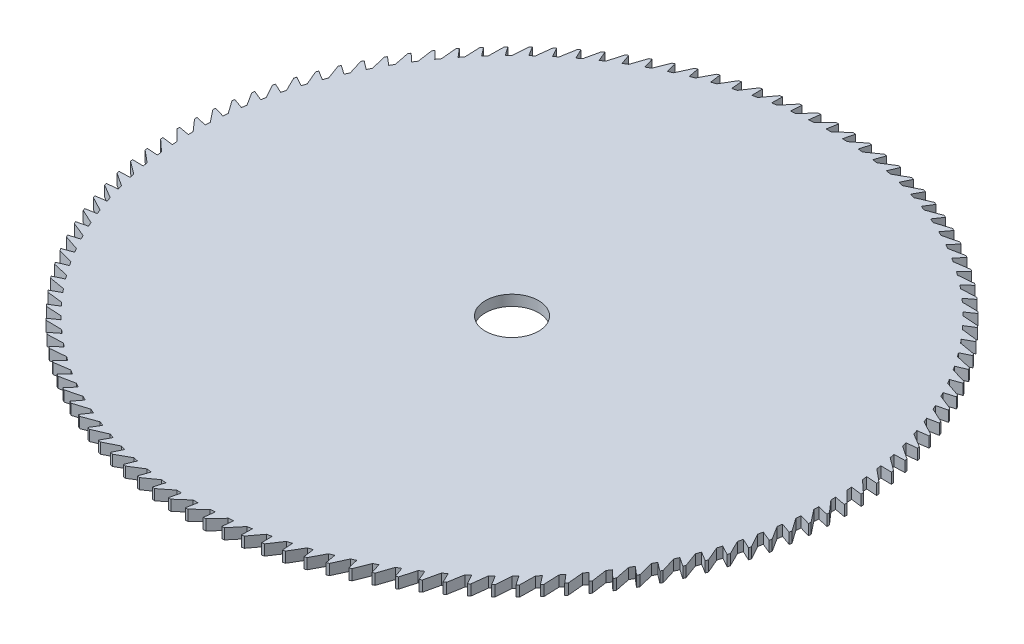
SolidWorks part; units mm, degrees
ref_plane "Front Plane" through (0, 0, 0) normal (0, 0, 1) x (1, 0, 0)
ref_plane "Top Plane" through (0, 0, 0) normal (0, 1, 0) x (1, 0, 0)
ref_plane "Right Plane" through (0, 0, 0) normal (1, 0, 0) x (0, 0, -1)
sketch "Sketch2" plane through (0, 0, 0) normal (0, 1, 0) x (1, 0, 0)
  circle A0 centre (0, 0) radius 150
  circle A1 centre (0, 0) radius 12.5
  dimension "D1" = 25
  dimension "D2" = 300
extrude "Boss-Extrude1" add sketch "Sketch2" along normal blind 5
sketch "Sketch3" plane through (0, 5, 0) normal (0, 1, 0) x (1, 0, 0)
  line L0 (0, 150) -> (0, -150) construction
  line L1 (0, 150) -> (5.59, 154.8992)
  line L2 (6.7665, 154.8522) -> (5.59, 149.8958)
  line L3 (7.8504, 149.7944) -> (13.6891, 154.3943)
  line L4 (14.8616, 154.2859) -> (13.4273, 149.3978)
  line L5 (15.6793, 149.1783) -> (21.7508, 153.4663)
  line L6 (22.9159, 153.2966) -> (21.2278, 148.4903)
  line L7 (23.4652, 148.1533) -> (29.7528, 152.1176)
  line L8 (30.9074, 151.8872) -> (28.9701, 147.1759)
  line L9 (31.1868, 146.7221) -> (37.6732, 150.352)
  line L10 (38.8142, 150.0615) -> (36.6329, 145.458)
  line L11 (38.8229, 144.8889) -> (45.4904, 148.1743)
  line L12 (46.6147, 147.8245) -> (44.1954, 143.3414)
  line L13 (46.3525, 142.6585) -> (53.1829, 145.5905)
  line L14 (54.2873, 145.1823) -> (51.6368, 140.832)
  line L15 (53.7552, 140.0371) -> (60.7296, 142.6076)
  line L16 (61.8112, 142.1421) -> (58.9366, 137.9365)
  line L17 (61.0105, 137.0318) -> (68.1099, 139.2338)
  line L18 (69.1656, 138.7124) -> (66.0748, 134.663)
  line L19 (68.0986, 133.651) -> (75.3035, 135.4784)
  line L20 (76.3304, 134.9024) -> (73.032, 131.0203)
  line L21 (75, 129.9038) -> (82.2907, 131.3516)
  line L22 (83.2861, 130.7227) -> (79.789, 127.0186)
  line L23 (81.6959, 125.8006) -> (89.0523, 126.8648)
  line L24 (90.0134, 126.1847) -> (86.3273, 122.6687)
  line L25 (88.1678, 121.3525) -> (95.5699, 122.0303)
  line L26 (96.4941, 121.3008) -> (92.629, 117.9825)
  line L27 (94.3981, 116.5719) -> (101.8255, 116.8614)
  line L28 (102.7102, 116.0845) -> (98.6767, 112.973)
  line L29 (100.3696, 111.4717) -> (107.802, 111.3721)
  line L30 (108.6449, 110.55) -> (104.4541, 107.6538)
  line L31 (106.066, 106.066) -> (113.483, 105.5775)
  line L32 (114.2817, 104.7124) -> (109.9451, 102.0396)
  line L33 (111.4717, 100.3696) -> (118.853, 99.4936)
  line L34 (119.6053, 98.5879) -> (115.1347, 96.1457)
  line L35 (116.5719, 94.3981) -> (123.8972, 93.137)
  line L36 (124.6011, 92.1931) -> (120.0088, 89.9882)
  line L37 (121.3525, 88.1678) -> (128.6018, 86.525)
  line L38 (129.2553, 85.5456) -> (124.554, 83.5841)
  line L39 (125.8006, 81.6959) -> (132.9539, 79.676)
  line L40 (133.5553, 78.6637) -> (128.7577, 76.9509)
  line L41 (129.9038, 75) -> (136.9416, 72.6085)
  line L42 (137.4892, 71.5662) -> (132.6086, 70.1068)
  line L43 (133.651, 68.0986) -> (140.554, 65.342)
  line L44 (141.0463, 64.2724) -> (136.0959, 63.0705)
  line L45 (137.0318, 61.0105) -> (143.7811, 57.8964)
  line L46 (144.2167, 56.8026) -> (139.2103, 55.8614)
  line L47 (140.0371, 53.7552) -> (146.6141, 50.2922)
  line L48 (146.9919, 49.177) -> (141.9431, 48.4991)
  line L49 (142.6585, 46.3525) -> (149.0453, 42.5501)
  line L50 (149.3642, 41.4166) -> (144.2868, 41.0039)
  line L51 (144.8889, 38.8229) -> (151.0679, 34.6913)
  line L52 (151.3271, 33.5428) -> (146.235, 33.3964)
  line L53 (146.7221, 31.1868) -> (152.6765, 26.7375)
  line L54 (152.8752, 25.5769) -> (147.7824, 25.6972)
  line L55 (148.1533, 23.4652) -> (153.8666, 18.7104)
  line L56 (154.0043, 17.541) -> (148.9248, 17.9277)
  line L57 (149.1783, 15.6793) -> (154.6349, 10.632)
  line L58 (154.7112, 9.457) -> (149.659, 10.109)
  line L59 (149.7944, 7.8504) -> (154.9794, 2.5244)
  line L60 (154.9941, 1.3471) -> (149.9829, 2.2626)
  line L61 (150, 0) -> (154.8992, -5.59)
  line L62 (154.8522, -6.7665) -> (149.8958, -5.59)
  line L63 (149.7944, -7.8504) -> (154.3943, -13.6891)
  line L64 (154.2859, -14.8616) -> (149.3978, -13.4273)
  line L65 (149.1783, -15.6793) -> (153.4663, -21.7508)
  line L66 (153.2966, -22.9159) -> (148.4903, -21.2278)
  line L67 (148.1533, -23.4652) -> (152.1176, -29.7528)
  line L68 (151.8872, -30.9074) -> (147.1759, -28.9701)
  line L69 (146.7221, -31.1868) -> (150.352, -37.6732)
  line L70 (150.0615, -38.8142) -> (145.458, -36.6329)
  line L71 (144.8889, -38.8229) -> (148.1743, -45.4904)
  line L72 (147.8245, -46.6147) -> (143.3414, -44.1954)
  line L73 (142.6585, -46.3525) -> (145.5905, -53.1829)
  line L74 (145.1823, -54.2873) -> (140.832, -51.6368)
  line L75 (140.0371, -53.7552) -> (142.6076, -60.7296)
  line L76 (142.1421, -61.8112) -> (137.9365, -58.9366)
  line L77 (137.0318, -61.0105) -> (139.2338, -68.1099)
  line L78 (138.7124, -69.1656) -> (134.663, -66.0748)
  line L79 (133.651, -68.0986) -> (135.4784, -75.3035)
  line L80 (134.9024, -76.3304) -> (131.0203, -73.032)
  line L81 (129.9038, -75) -> (131.3516, -82.2907)
  line L82 (130.7227, -83.2861) -> (127.0186, -79.789)
  line L83 (125.8006, -81.6959) -> (126.8648, -89.0523)
  line L84 (126.1847, -90.0134) -> (122.6687, -86.3273)
  line L85 (121.3525, -88.1678) -> (122.0303, -95.5699)
  line L86 (121.3008, -96.4941) -> (117.9825, -92.629)
  line L87 (116.5719, -94.3981) -> (116.8614, -101.8255)
  line L88 (116.0845, -102.7102) -> (112.973, -98.6767)
  line L89 (111.4717, -100.3696) -> (111.3721, -107.802)
  line L90 (110.55, -108.6449) -> (107.6538, -104.4541)
  line L91 (106.066, -106.066) -> (105.5775, -113.483)
  line L92 (104.7124, -114.2817) -> (102.0396, -109.9451)
  line L93 (100.3696, -111.4717) -> (99.4936, -118.853)
  line L94 (98.5879, -119.6053) -> (96.1457, -115.1347)
  line L95 (94.3981, -116.5719) -> (93.137, -123.8972)
  line L96 (92.1931, -124.6011) -> (89.9882, -120.0088)
  line L97 (88.1678, -121.3525) -> (86.525, -128.6018)
  line L98 (85.5456, -129.2553) -> (83.5841, -124.554)
  line L99 (81.6959, -125.8006) -> (79.676, -132.9539)
  line L100 (78.6637, -133.5553) -> (76.9509, -128.7577)
  line L101 (75, -129.9038) -> (72.6085, -136.9416)
  line L102 (71.5662, -137.4892) -> (70.1068, -132.6086)
  line L103 (68.0986, -133.651) -> (65.342, -140.554)
  line L104 (64.2724, -141.0463) -> (63.0705, -136.0959)
  line L105 (61.0105, -137.0318) -> (57.8964, -143.7811)
  line L106 (56.8026, -144.2167) -> (55.8614, -139.2103)
  line L107 (53.7552, -140.0371) -> (50.2922, -146.6141)
  line L108 (49.177, -146.9919) -> (48.4991, -141.9431)
  line L109 (46.3525, -142.6585) -> (42.5501, -149.0453)
  line L110 (41.4166, -149.3642) -> (41.0039, -144.2868)
  line L111 (38.8229, -144.8889) -> (34.6913, -151.0679)
  line L112 (33.5428, -151.3271) -> (33.3964, -146.235)
  line L113 (31.1868, -146.7221) -> (26.7375, -152.6765)
  line L114 (25.5769, -152.8752) -> (25.6972, -147.7824)
  line L115 (23.4652, -148.1533) -> (18.7104, -153.8666)
  line L116 (17.541, -154.0043) -> (17.9277, -148.9248)
  line L117 (15.6793, -149.1783) -> (10.632, -154.6349)
  line L118 (9.457, -154.7112) -> (10.109, -149.659)
  line L119 (7.8504, -149.7944) -> (2.5244, -154.9794)
  line L120 (1.3471, -154.9941) -> (2.2626, -149.9829)
  line L121 (0, -150) -> (-5.59, -154.8992)
  line L122 (-6.7665, -154.8522) -> (-5.59, -149.8958)
  line L123 (-7.8504, -149.7944) -> (-13.6891, -154.3943)
  line L124 (-14.8616, -154.2859) -> (-13.4273, -149.3978)
  line L125 (-15.6793, -149.1783) -> (-21.7508, -153.4663)
  line L126 (-22.9159, -153.2966) -> (-21.2278, -148.4903)
  line L127 (-23.4652, -148.1533) -> (-29.7528, -152.1176)
  line L128 (-30.9074, -151.8872) -> (-28.9701, -147.1759)
  line L129 (-31.1868, -146.7221) -> (-37.6732, -150.352)
  line L130 (-38.8142, -150.0615) -> (-36.6329, -145.458)
  line L131 (-38.8229, -144.8889) -> (-45.4904, -148.1743)
  line L132 (-46.6147, -147.8245) -> (-44.1954, -143.3414)
  line L133 (-46.3525, -142.6585) -> (-53.1829, -145.5905)
  line L134 (-54.2873, -145.1823) -> (-51.6368, -140.832)
  line L135 (-53.7552, -140.0371) -> (-60.7296, -142.6076)
  line L136 (-61.8112, -142.1421) -> (-58.9366, -137.9365)
  line L137 (-61.0105, -137.0318) -> (-68.1099, -139.2338)
  line L138 (-69.1656, -138.7124) -> (-66.0748, -134.663)
  line L139 (-68.0986, -133.651) -> (-75.3035, -135.4784)
  line L140 (-76.3304, -134.9024) -> (-73.032, -131.0203)
  line L141 (-75, -129.9038) -> (-82.2907, -131.3516)
  line L142 (-83.2861, -130.7227) -> (-79.789, -127.0186)
  line L143 (-81.6959, -125.8006) -> (-89.0523, -126.8648)
  line L144 (-90.0134, -126.1847) -> (-86.3273, -122.6687)
  line L145 (-88.1678, -121.3525) -> (-95.5699, -122.0303)
  line L146 (-96.4941, -121.3008) -> (-92.629, -117.9825)
  line L147 (-94.3981, -116.5719) -> (-101.8255, -116.8614)
  line L148 (-102.7102, -116.0845) -> (-98.6767, -112.973)
  line L149 (-100.3696, -111.4717) -> (-107.802, -111.3721)
  line L150 (-108.6449, -110.55) -> (-104.4541, -107.6538)
  line L151 (-106.066, -106.066) -> (-113.483, -105.5775)
  line L152 (-114.2817, -104.7124) -> (-109.9451, -102.0396)
  line L153 (-111.4717, -100.3696) -> (-118.853, -99.4936)
  line L154 (-119.6053, -98.5879) -> (-115.1347, -96.1457)
  line L155 (-116.5719, -94.3981) -> (-123.8972, -93.137)
  line L156 (-124.6011, -92.1931) -> (-120.0088, -89.9882)
  line L157 (-121.3525, -88.1678) -> (-128.6018, -86.525)
  line L158 (-129.2553, -85.5456) -> (-124.554, -83.5841)
  line L159 (-125.8006, -81.6959) -> (-132.9539, -79.676)
  line L160 (-133.5553, -78.6637) -> (-128.7577, -76.9509)
  line L161 (-129.9038, -75) -> (-136.9416, -72.6085)
  line L162 (-137.4892, -71.5662) -> (-132.6086, -70.1068)
  line L163 (-133.651, -68.0986) -> (-140.554, -65.342)
  line L164 (-141.0463, -64.2724) -> (-136.0959, -63.0705)
  line L165 (-137.0318, -61.0105) -> (-143.7811, -57.8964)
  line L166 (-144.2167, -56.8026) -> (-139.2103, -55.8614)
  line L167 (-140.0371, -53.7552) -> (-146.6141, -50.2922)
  line L168 (-146.9919, -49.177) -> (-141.9431, -48.4991)
  line L169 (-142.6585, -46.3525) -> (-149.0453, -42.5501)
  line L170 (-149.3642, -41.4166) -> (-144.2868, -41.0039)
  line L171 (-144.8889, -38.8229) -> (-151.0679, -34.6913)
  line L172 (-151.3271, -33.5428) -> (-146.235, -33.3964)
  line L173 (-146.7221, -31.1868) -> (-152.6765, -26.7375)
  line L174 (-152.8752, -25.5769) -> (-147.7824, -25.6972)
  line L175 (-148.1533, -23.4652) -> (-153.8666, -18.7104)
  line L176 (-154.0043, -17.541) -> (-148.9248, -17.9277)
  line L177 (-149.1783, -15.6793) -> (-154.6349, -10.632)
  line L178 (-154.7112, -9.457) -> (-149.659, -10.109)
  line L179 (-149.7944, -7.8504) -> (-154.9794, -2.5244)
  line L180 (-154.9941, -1.3471) -> (-149.9829, -2.2626)
  line L181 (-150, 0) -> (-154.8992, 5.59)
  line L182 (-154.8522, 6.7665) -> (-149.8958, 5.59)
  line L183 (-149.7944, 7.8504) -> (-154.3943, 13.6891)
  line L184 (-154.2859, 14.8616) -> (-149.3978, 13.4273)
  line L185 (-149.1783, 15.6793) -> (-153.4663, 21.7508)
  line L186 (-153.2966, 22.9159) -> (-148.4903, 21.2278)
  line L187 (-148.1533, 23.4652) -> (-152.1176, 29.7528)
  line L188 (-151.8872, 30.9074) -> (-147.1759, 28.9701)
  line L189 (-146.7221, 31.1868) -> (-150.352, 37.6732)
  line L190 (-150.0615, 38.8142) -> (-145.458, 36.6329)
  line L191 (-144.8889, 38.8229) -> (-148.1743, 45.4904)
  line L192 (-147.8245, 46.6147) -> (-143.3414, 44.1954)
  line L193 (-142.6585, 46.3525) -> (-145.5905, 53.1829)
  line L194 (-145.1823, 54.2873) -> (-140.832, 51.6368)
  line L195 (-140.0371, 53.7552) -> (-142.6076, 60.7296)
  line L196 (-142.1421, 61.8112) -> (-137.9365, 58.9366)
  line L197 (-137.0318, 61.0105) -> (-139.2338, 68.1099)
  line L198 (-138.7124, 69.1656) -> (-134.663, 66.0748)
  line L199 (-133.651, 68.0986) -> (-135.4784, 75.3035)
  line L200 (-134.9024, 76.3304) -> (-131.0203, 73.032)
  line L201 (-129.9038, 75) -> (-131.3516, 82.2907)
  line L202 (-130.7227, 83.2861) -> (-127.0186, 79.789)
  line L203 (-125.8006, 81.6959) -> (-126.8648, 89.0523)
  line L204 (-126.1847, 90.0134) -> (-122.6687, 86.3273)
  line L205 (-121.3525, 88.1678) -> (-122.0303, 95.5699)
  line L206 (-121.3008, 96.4941) -> (-117.9825, 92.629)
  line L207 (-116.5719, 94.3981) -> (-116.8614, 101.8255)
  line L208 (-116.0845, 102.7102) -> (-112.973, 98.6767)
  line L209 (-111.4717, 100.3696) -> (-111.3721, 107.802)
  line L210 (-110.55, 108.6449) -> (-107.6538, 104.4541)
  line L211 (-106.066, 106.066) -> (-105.5775, 113.483)
  line L212 (-104.7124, 114.2817) -> (-102.0396, 109.9451)
  line L213 (-100.3696, 111.4717) -> (-99.4936, 118.853)
  line L214 (-98.5879, 119.6053) -> (-96.1457, 115.1347)
  line L215 (-94.3981, 116.5719) -> (-93.137, 123.8972)
  line L216 (-92.1931, 124.6011) -> (-89.9882, 120.0088)
  line L217 (-88.1678, 121.3525) -> (-86.525, 128.6018)
  line L218 (-85.5456, 129.2553) -> (-83.5841, 124.554)
  line L219 (-81.6959, 125.8006) -> (-79.676, 132.9539)
  line L220 (-78.6637, 133.5553) -> (-76.9509, 128.7577)
  line L221 (-75, 129.9038) -> (-72.6085, 136.9416)
  line L222 (-71.5662, 137.4892) -> (-70.1068, 132.6086)
  line L223 (-68.0986, 133.651) -> (-65.342, 140.554)
  line L224 (-64.2724, 141.0463) -> (-63.0705, 136.0959)
  line L225 (-61.0105, 137.0318) -> (-57.8964, 143.7811)
  line L226 (-56.8026, 144.2167) -> (-55.8614, 139.2103)
  line L227 (-53.7552, 140.0371) -> (-50.2922, 146.6141)
  line L228 (-49.177, 146.9919) -> (-48.4991, 141.9431)
  line L229 (-46.3525, 142.6585) -> (-42.5501, 149.0453)
  line L230 (-41.4166, 149.3642) -> (-41.0039, 144.2868)
  line L231 (-38.8229, 144.8889) -> (-34.6913, 151.0679)
  line L232 (-33.5428, 151.3271) -> (-33.3964, 146.235)
  line L233 (-31.1868, 146.7221) -> (-26.7375, 152.6765)
  line L234 (-25.5769, 152.8752) -> (-25.6972, 147.7824)
  line L235 (-23.4652, 148.1533) -> (-18.7104, 153.8666)
  line L236 (-17.541, 154.0043) -> (-17.9277, 148.9248)
  line L237 (-15.6793, 149.1783) -> (-10.632, 154.6349)
  line L238 (-9.457, 154.7112) -> (-10.109, 149.659)
  line L239 (-7.8504, 149.7944) -> (-2.5244, 154.9794)
  line L240 (-1.3471, 154.9941) -> (-2.2626, 149.9829)
  circle A0 centre (0, 0) radius 150 construction
  arc A1 (6.7665, 154.8522) -> (5.59, 154.8992) centre (0, 0) ccw
  arc A2 (5.59, 149.8958) -> (0, 150) centre (0, 0) ccw
  arc A3 (14.8616, 154.2859) -> (13.6891, 154.3943) centre (0, 0) ccw
  arc A4 (13.4273, 149.3978) -> (7.8504, 149.7944) centre (0, 0) ccw
  arc A5 (22.9159, 153.2966) -> (21.7508, 153.4663) centre (0, 0) ccw
  arc A6 (21.2278, 148.4903) -> (15.6793, 149.1783) centre (0, 0) ccw
  arc A7 (30.9074, 151.8872) -> (29.7528, 152.1176) centre (0, 0) ccw
  arc A8 (28.9701, 147.1759) -> (23.4652, 148.1533) centre (0, 0) ccw
  arc A9 (38.8142, 150.0615) -> (37.6732, 150.352) centre (0, 0) ccw
  arc A10 (36.6329, 145.458) -> (31.1868, 146.7221) centre (0, 0) ccw
  arc A11 (46.6147, 147.8245) -> (45.4904, 148.1743) centre (0, 0) ccw
  arc A12 (44.1954, 143.3414) -> (38.8229, 144.8889) centre (0, 0) ccw
  arc A13 (54.2873, 145.1823) -> (53.1829, 145.5905) centre (0, 0) ccw
  arc A14 (51.6368, 140.832) -> (46.3525, 142.6585) centre (0, 0) ccw
  arc A15 (61.8112, 142.1421) -> (60.7296, 142.6076) centre (0, 0) ccw
  arc A16 (58.9366, 137.9365) -> (53.7552, 140.0371) centre (0, 0) ccw
  arc A17 (69.1656, 138.7124) -> (68.1099, 139.2338) centre (0, 0) ccw
  arc A18 (66.0748, 134.663) -> (61.0105, 137.0318) centre (0, 0) ccw
  arc A19 (76.3304, 134.9024) -> (75.3035, 135.4784) centre (0, 0) ccw
  arc A20 (73.032, 131.0203) -> (68.0986, 133.651) centre (0, 0) ccw
  arc A21 (83.2861, 130.7227) -> (82.2907, 131.3516) centre (0, 0) ccw
  arc A22 (79.789, 127.0186) -> (75, 129.9038) centre (0, 0) ccw
  arc A23 (90.0134, 126.1847) -> (89.0523, 126.8648) centre (0, 0) ccw
  arc A24 (86.3273, 122.6687) -> (81.6959, 125.8006) centre (0, 0) ccw
  arc A25 (96.4941, 121.3008) -> (95.5699, 122.0303) centre (0, 0) ccw
  arc A26 (92.629, 117.9825) -> (88.1678, 121.3525) centre (0, 0) ccw
  arc A27 (102.7102, 116.0845) -> (101.8255, 116.8614) centre (0, 0) ccw
  arc A28 (98.6767, 112.973) -> (94.3981, 116.5719) centre (0, 0) ccw
  arc A29 (108.6449, 110.55) -> (107.802, 111.3721) centre (0, 0) ccw
  arc A30 (104.4541, 107.6538) -> (100.3696, 111.4717) centre (0, 0) ccw
  arc A31 (114.2817, 104.7124) -> (113.483, 105.5775) centre (0, 0) ccw
  arc A32 (109.9451, 102.0396) -> (106.066, 106.066) centre (0, 0) ccw
  arc A33 (119.6053, 98.5879) -> (118.853, 99.4936) centre (0, 0) ccw
  arc A34 (115.1347, 96.1457) -> (111.4717, 100.3696) centre (0, 0) ccw
  arc A35 (124.6011, 92.1931) -> (123.8972, 93.137) centre (0, 0) ccw
  arc A36 (120.0088, 89.9882) -> (116.5719, 94.3981) centre (0, 0) ccw
  arc A37 (129.2553, 85.5456) -> (128.6018, 86.525) centre (0, 0) ccw
  arc A38 (124.554, 83.5841) -> (121.3525, 88.1678) centre (0, 0) ccw
  arc A39 (133.5553, 78.6637) -> (132.9539, 79.676) centre (0, 0) ccw
  arc A40 (128.7577, 76.9509) -> (125.8006, 81.6959) centre (0, 0) ccw
  arc A41 (137.4892, 71.5662) -> (136.9416, 72.6085) centre (0, 0) ccw
  arc A42 (132.6086, 70.1068) -> (129.9038, 75) centre (0, 0) ccw
  arc A43 (141.0463, 64.2724) -> (140.554, 65.342) centre (0, 0) ccw
  arc A44 (136.0959, 63.0705) -> (133.651, 68.0986) centre (0, 0) ccw
  arc A45 (144.2167, 56.8026) -> (143.7811, 57.8964) centre (0, 0) ccw
  arc A46 (139.2103, 55.8614) -> (137.0318, 61.0105) centre (0, 0) ccw
  arc A47 (146.9919, 49.177) -> (146.6141, 50.2922) centre (0, 0) ccw
  arc A48 (141.9431, 48.4991) -> (140.0371, 53.7552) centre (0, 0) ccw
  arc A49 (149.3642, 41.4166) -> (149.0453, 42.5501) centre (0, 0) ccw
  arc A50 (144.2868, 41.0039) -> (142.6585, 46.3525) centre (0, 0) ccw
  arc A51 (151.3271, 33.5428) -> (151.0679, 34.6913) centre (0, 0) ccw
  arc A52 (146.235, 33.3964) -> (144.8889, 38.8229) centre (0, 0) ccw
  arc A53 (152.8752, 25.5769) -> (152.6765, 26.7375) centre (0, 0) ccw
  arc A54 (147.7824, 25.6972) -> (146.7221, 31.1868) centre (0, 0) ccw
  arc A55 (154.0043, 17.541) -> (153.8666, 18.7104) centre (0, 0) ccw
  arc A56 (148.9248, 17.9277) -> (148.1533, 23.4652) centre (0, 0) ccw
  arc A57 (154.7112, 9.457) -> (154.6349, 10.632) centre (0, 0) ccw
  arc A58 (149.659, 10.109) -> (149.1783, 15.6793) centre (0, 0) ccw
  arc A59 (154.9941, 1.3471) -> (154.9794, 2.5244) centre (0, 0) ccw
  arc A60 (149.9829, 2.2626) -> (149.7944, 7.8504) centre (0, 0) ccw
  arc A61 (154.8522, -6.7665) -> (154.8992, -5.59) centre (0, 0) ccw
  arc A62 (149.8958, -5.59) -> (150, 0) centre (0, 0) ccw
  arc A63 (154.2859, -14.8616) -> (154.3943, -13.6891) centre (0, 0) ccw
  arc A64 (149.3978, -13.4273) -> (149.7944, -7.8504) centre (0, 0) ccw
  arc A65 (153.2966, -22.9159) -> (153.4663, -21.7508) centre (0, 0) ccw
  arc A66 (148.4903, -21.2278) -> (149.1783, -15.6793) centre (0, 0) ccw
  arc A67 (151.8872, -30.9074) -> (152.1176, -29.7528) centre (0, 0) ccw
  arc A68 (147.1759, -28.9701) -> (148.1533, -23.4652) centre (0, 0) ccw
  arc A69 (150.0615, -38.8142) -> (150.352, -37.6732) centre (0, 0) ccw
  arc A70 (145.458, -36.6329) -> (146.7221, -31.1868) centre (0, 0) ccw
  arc A71 (147.8245, -46.6147) -> (148.1743, -45.4904) centre (0, 0) ccw
  arc A72 (143.3414, -44.1954) -> (144.8889, -38.8229) centre (0, 0) ccw
  arc A73 (145.1823, -54.2873) -> (145.5905, -53.1829) centre (0, 0) ccw
  arc A74 (140.832, -51.6368) -> (142.6585, -46.3525) centre (0, 0) ccw
  arc A75 (142.1421, -61.8112) -> (142.6076, -60.7296) centre (0, 0) ccw
  arc A76 (137.9365, -58.9366) -> (140.0371, -53.7552) centre (0, 0) ccw
  arc A77 (138.7124, -69.1656) -> (139.2338, -68.1099) centre (0, 0) ccw
  arc A78 (134.663, -66.0748) -> (137.0318, -61.0105) centre (0, 0) ccw
  arc A79 (134.9024, -76.3304) -> (135.4784, -75.3035) centre (0, 0) ccw
  arc A80 (131.0203, -73.032) -> (133.651, -68.0986) centre (0, 0) ccw
  arc A81 (130.7227, -83.2861) -> (131.3516, -82.2907) centre (0, 0) ccw
  arc A82 (127.0186, -79.789) -> (129.9038, -75) centre (0, 0) ccw
  arc A83 (126.1847, -90.0134) -> (126.8648, -89.0523) centre (0, 0) ccw
  arc A84 (122.6687, -86.3273) -> (125.8006, -81.6959) centre (0, 0) ccw
  arc A85 (121.3008, -96.4941) -> (122.0303, -95.5699) centre (0, 0) ccw
  arc A86 (117.9825, -92.629) -> (121.3525, -88.1678) centre (0, 0) ccw
  arc A87 (116.0845, -102.7102) -> (116.8614, -101.8255) centre (0, 0) ccw
  arc A88 (112.973, -98.6767) -> (116.5719, -94.3981) centre (0, 0) ccw
  arc A89 (110.55, -108.6449) -> (111.3721, -107.802) centre (0, 0) ccw
  arc A90 (107.6538, -104.4541) -> (111.4717, -100.3696) centre (0, 0) ccw
  arc A91 (104.7124, -114.2817) -> (105.5775, -113.483) centre (0, 0) ccw
  arc A92 (102.0396, -109.9451) -> (106.066, -106.066) centre (0, 0) ccw
  arc A93 (98.5879, -119.6053) -> (99.4936, -118.853) centre (0, 0) ccw
  arc A94 (96.1457, -115.1347) -> (100.3696, -111.4717) centre (0, 0) ccw
  arc A95 (92.1931, -124.6011) -> (93.137, -123.8972) centre (0, 0) ccw
  arc A96 (89.9882, -120.0088) -> (94.3981, -116.5719) centre (0, 0) ccw
  arc A97 (85.5456, -129.2553) -> (86.525, -128.6018) centre (0, 0) ccw
  arc A98 (83.5841, -124.554) -> (88.1678, -121.3525) centre (0, 0) ccw
  arc A99 (78.6637, -133.5553) -> (79.676, -132.9539) centre (0, 0) ccw
  arc A100 (76.9509, -128.7577) -> (81.6959, -125.8006) centre (0, 0) ccw
  arc A101 (71.5662, -137.4892) -> (72.6085, -136.9416) centre (0, 0) ccw
  arc A102 (70.1068, -132.6086) -> (75, -129.9038) centre (0, 0) ccw
  arc A103 (64.2724, -141.0463) -> (65.342, -140.554) centre (0, 0) ccw
  arc A104 (63.0705, -136.0959) -> (68.0986, -133.651) centre (0, 0) ccw
  arc A105 (56.8026, -144.2167) -> (57.8964, -143.7811) centre (0, 0) ccw
  arc A106 (55.8614, -139.2103) -> (61.0105, -137.0318) centre (0, 0) ccw
  arc A107 (49.177, -146.9919) -> (50.2922, -146.6141) centre (0, 0) ccw
  arc A108 (48.4991, -141.9431) -> (53.7552, -140.0371) centre (0, 0) ccw
  arc A109 (41.4166, -149.3642) -> (42.5501, -149.0453) centre (0, 0) ccw
  arc A110 (41.0039, -144.2868) -> (46.3525, -142.6585) centre (0, 0) ccw
  arc A111 (33.5428, -151.3271) -> (34.6913, -151.0679) centre (0, 0) ccw
  arc A112 (33.3964, -146.235) -> (38.8229, -144.8889) centre (0, 0) ccw
  arc A113 (25.5769, -152.8752) -> (26.7375, -152.6765) centre (0, 0) ccw
  arc A114 (25.6972, -147.7824) -> (31.1868, -146.7221) centre (0, 0) ccw
  arc A115 (17.541, -154.0043) -> (18.7104, -153.8666) centre (0, 0) ccw
  arc A116 (17.9277, -148.9248) -> (23.4652, -148.1533) centre (0, 0) ccw
  arc A117 (9.457, -154.7112) -> (10.632, -154.6349) centre (0, 0) ccw
  arc A118 (10.109, -149.659) -> (15.6793, -149.1783) centre (0, 0) ccw
  arc A119 (1.3471, -154.9941) -> (2.5244, -154.9794) centre (0, 0) ccw
  arc A120 (2.2626, -149.9829) -> (7.8504, -149.7944) centre (0, 0) ccw
  arc A121 (-6.7665, -154.8522) -> (-5.59, -154.8992) centre (0, 0) ccw
  arc A122 (-5.59, -149.8958) -> (0, -150) centre (0, 0) ccw
  arc A123 (-14.8616, -154.2859) -> (-13.6891, -154.3943) centre (0, 0) ccw
  arc A124 (-13.4273, -149.3978) -> (-7.8504, -149.7944) centre (0, 0) ccw
  arc A125 (-22.9159, -153.2966) -> (-21.7508, -153.4663) centre (0, 0) ccw
  arc A126 (-21.2278, -148.4903) -> (-15.6793, -149.1783) centre (0, 0) ccw
  arc A127 (-30.9074, -151.8872) -> (-29.7528, -152.1176) centre (0, 0) ccw
  arc A128 (-28.9701, -147.1759) -> (-23.4652, -148.1533) centre (0, 0) ccw
  arc A129 (-38.8142, -150.0615) -> (-37.6732, -150.352) centre (0, 0) ccw
  arc A130 (-36.6329, -145.458) -> (-31.1868, -146.7221) centre (0, 0) ccw
  arc A131 (-46.6147, -147.8245) -> (-45.4904, -148.1743) centre (0, 0) ccw
  arc A132 (-44.1954, -143.3414) -> (-38.8229, -144.8889) centre (0, 0) ccw
  arc A133 (-54.2873, -145.1823) -> (-53.1829, -145.5905) centre (0, 0) ccw
  arc A134 (-51.6368, -140.832) -> (-46.3525, -142.6585) centre (0, 0) ccw
  arc A135 (-61.8112, -142.1421) -> (-60.7296, -142.6076) centre (0, 0) ccw
  arc A136 (-58.9366, -137.9365) -> (-53.7552, -140.0371) centre (0, 0) ccw
  arc A137 (-69.1656, -138.7124) -> (-68.1099, -139.2338) centre (0, 0) ccw
  arc A138 (-66.0748, -134.663) -> (-61.0105, -137.0318) centre (0, 0) ccw
  arc A139 (-76.3304, -134.9024) -> (-75.3035, -135.4784) centre (0, 0) ccw
  arc A140 (-73.032, -131.0203) -> (-68.0986, -133.651) centre (0, 0) ccw
  arc A141 (-83.2861, -130.7227) -> (-82.2907, -131.3516) centre (0, 0) ccw
  arc A142 (-79.789, -127.0186) -> (-75, -129.9038) centre (0, 0) ccw
  arc A143 (-90.0134, -126.1847) -> (-89.0523, -126.8648) centre (0, 0) ccw
  arc A144 (-86.3273, -122.6687) -> (-81.6959, -125.8006) centre (0, 0) ccw
  arc A145 (-96.4941, -121.3008) -> (-95.5699, -122.0303) centre (0, 0) ccw
  arc A146 (-92.629, -117.9825) -> (-88.1678, -121.3525) centre (0, 0) ccw
  arc A147 (-102.7102, -116.0845) -> (-101.8255, -116.8614) centre (0, 0) ccw
  arc A148 (-98.6767, -112.973) -> (-94.3981, -116.5719) centre (0, 0) ccw
  arc A149 (-108.6449, -110.55) -> (-107.802, -111.3721) centre (0, 0) ccw
  arc A150 (-104.4541, -107.6538) -> (-100.3696, -111.4717) centre (0, 0) ccw
  arc A151 (-114.2817, -104.7124) -> (-113.483, -105.5775) centre (0, 0) ccw
  arc A152 (-109.9451, -102.0396) -> (-106.066, -106.066) centre (0, 0) ccw
  arc A153 (-119.6053, -98.5879) -> (-118.853, -99.4936) centre (0, 0) ccw
  arc A154 (-115.1347, -96.1457) -> (-111.4717, -100.3696) centre (0, 0) ccw
  arc A155 (-124.6011, -92.1931) -> (-123.8972, -93.137) centre (0, 0) ccw
  arc A156 (-120.0088, -89.9882) -> (-116.5719, -94.3981) centre (0, 0) ccw
  arc A157 (-129.2553, -85.5456) -> (-128.6018, -86.525) centre (0, 0) ccw
  arc A158 (-124.554, -83.5841) -> (-121.3525, -88.1678) centre (0, 0) ccw
  arc A159 (-133.5553, -78.6637) -> (-132.9539, -79.676) centre (0, 0) ccw
  arc A160 (-128.7577, -76.9509) -> (-125.8006, -81.6959) centre (0, 0) ccw
  arc A161 (-137.4892, -71.5662) -> (-136.9416, -72.6085) centre (0, 0) ccw
  arc A162 (-132.6086, -70.1068) -> (-129.9038, -75) centre (0, 0) ccw
  arc A163 (-141.0463, -64.2724) -> (-140.554, -65.342) centre (0, 0) ccw
  arc A164 (-136.0959, -63.0705) -> (-133.651, -68.0986) centre (0, 0) ccw
  arc A165 (-144.2167, -56.8026) -> (-143.7811, -57.8964) centre (0, 0) ccw
  arc A166 (-139.2103, -55.8614) -> (-137.0318, -61.0105) centre (0, 0) ccw
  arc A167 (-146.9919, -49.177) -> (-146.6141, -50.2922) centre (0, 0) ccw
  arc A168 (-141.9431, -48.4991) -> (-140.0371, -53.7552) centre (0, 0) ccw
  arc A169 (-149.3642, -41.4166) -> (-149.0453, -42.5501) centre (0, 0) ccw
  arc A170 (-144.2868, -41.0039) -> (-142.6585, -46.3525) centre (0, 0) ccw
  arc A171 (-151.3271, -33.5428) -> (-151.0679, -34.6913) centre (0, 0) ccw
  arc A172 (-146.235, -33.3964) -> (-144.8889, -38.8229) centre (0, 0) ccw
  arc A173 (-152.8752, -25.5769) -> (-152.6765, -26.7375) centre (0, 0) ccw
  arc A174 (-147.7824, -25.6972) -> (-146.7221, -31.1868) centre (0, 0) ccw
  arc A175 (-154.0043, -17.541) -> (-153.8666, -18.7104) centre (0, 0) ccw
  arc A176 (-148.9248, -17.9277) -> (-148.1533, -23.4652) centre (0, 0) ccw
  arc A177 (-154.7112, -9.457) -> (-154.6349, -10.632) centre (0, 0) ccw
  arc A178 (-149.659, -10.109) -> (-149.1783, -15.6793) centre (0, 0) ccw
  arc A179 (-154.9941, -1.3471) -> (-154.9794, -2.5244) centre (0, 0) ccw
  arc A180 (-149.9829, -2.2626) -> (-149.7944, -7.8504) centre (0, 0) ccw
  arc A181 (-154.8522, 6.7665) -> (-154.8992, 5.59) centre (0, 0) ccw
  arc A182 (-149.8958, 5.59) -> (-150, 0) centre (0, 0) ccw
  arc A183 (-154.2859, 14.8616) -> (-154.3943, 13.6891) centre (0, 0) ccw
  arc A184 (-149.3978, 13.4273) -> (-149.7944, 7.8504) centre (0, 0) ccw
  arc A185 (-153.2966, 22.9159) -> (-153.4663, 21.7508) centre (0, 0) ccw
  arc A186 (-148.4903, 21.2278) -> (-149.1783, 15.6793) centre (0, 0) ccw
  arc A187 (-151.8872, 30.9074) -> (-152.1176, 29.7528) centre (0, 0) ccw
  arc A188 (-147.1759, 28.9701) -> (-148.1533, 23.4652) centre (0, 0) ccw
  arc A189 (-150.0615, 38.8142) -> (-150.352, 37.6732) centre (0, 0) ccw
  arc A190 (-145.458, 36.6329) -> (-146.7221, 31.1868) centre (0, 0) ccw
  arc A191 (-147.8245, 46.6147) -> (-148.1743, 45.4904) centre (0, 0) ccw
  arc A192 (-143.3414, 44.1954) -> (-144.8889, 38.8229) centre (0, 0) ccw
  arc A193 (-145.1823, 54.2873) -> (-145.5905, 53.1829) centre (0, 0) ccw
  arc A194 (-140.832, 51.6368) -> (-142.6585, 46.3525) centre (0, 0) ccw
  arc A195 (-142.1421, 61.8112) -> (-142.6076, 60.7296) centre (0, 0) ccw
  arc A196 (-137.9365, 58.9366) -> (-140.0371, 53.7552) centre (0, 0) ccw
  arc A197 (-138.7124, 69.1656) -> (-139.2338, 68.1099) centre (0, 0) ccw
  arc A198 (-134.663, 66.0748) -> (-137.0318, 61.0105) centre (0, 0) ccw
  arc A199 (-134.9024, 76.3304) -> (-135.4784, 75.3035) centre (0, 0) ccw
  arc A200 (-131.0203, 73.032) -> (-133.651, 68.0986) centre (0, 0) ccw
  arc A201 (-130.7227, 83.2861) -> (-131.3516, 82.2907) centre (0, 0) ccw
  arc A202 (-127.0186, 79.789) -> (-129.9038, 75) centre (0, 0) ccw
  arc A203 (-126.1847, 90.0134) -> (-126.8648, 89.0523) centre (0, 0) ccw
  arc A204 (-122.6687, 86.3273) -> (-125.8006, 81.6959) centre (0, 0) ccw
  arc A205 (-121.3008, 96.4941) -> (-122.0303, 95.5699) centre (0, 0) ccw
  arc A206 (-117.9825, 92.629) -> (-121.3525, 88.1678) centre (0, 0) ccw
  arc A207 (-116.0845, 102.7102) -> (-116.8614, 101.8255) centre (0, 0) ccw
  arc A208 (-112.973, 98.6767) -> (-116.5719, 94.3981) centre (0, 0) ccw
  arc A209 (-110.55, 108.6449) -> (-111.3721, 107.802) centre (0, 0) ccw
  arc A210 (-107.6538, 104.4541) -> (-111.4717, 100.3696) centre (0, 0) ccw
  arc A211 (-104.7124, 114.2817) -> (-105.5775, 113.483) centre (0, 0) ccw
  arc A212 (-102.0396, 109.9451) -> (-106.066, 106.066) centre (0, 0) ccw
  arc A213 (-98.5879, 119.6053) -> (-99.4936, 118.853) centre (0, 0) ccw
  arc A214 (-96.1457, 115.1347) -> (-100.3696, 111.4717) centre (0, 0) ccw
  arc A215 (-92.1931, 124.6011) -> (-93.137, 123.8972) centre (0, 0) ccw
  arc A216 (-89.9882, 120.0088) -> (-94.3981, 116.5719) centre (0, 0) ccw
  arc A217 (-85.5456, 129.2553) -> (-86.525, 128.6018) centre (0, 0) ccw
  arc A218 (-83.5841, 124.554) -> (-88.1678, 121.3525) centre (0, 0) ccw
  arc A219 (-78.6637, 133.5553) -> (-79.676, 132.9539) centre (0, 0) ccw
  arc A220 (-76.9509, 128.7577) -> (-81.6959, 125.8006) centre (0, 0) ccw
  arc A221 (-71.5662, 137.4892) -> (-72.6085, 136.9416) centre (0, 0) ccw
  arc A222 (-70.1068, 132.6086) -> (-75, 129.9038) centre (0, 0) ccw
  arc A223 (-64.2724, 141.0463) -> (-65.342, 140.554) centre (0, 0) ccw
  arc A224 (-63.0705, 136.0959) -> (-68.0986, 133.651) centre (0, 0) ccw
  arc A225 (-56.8026, 144.2167) -> (-57.8964, 143.7811) centre (0, 0) ccw
  arc A226 (-55.8614, 139.2103) -> (-61.0105, 137.0318) centre (0, 0) ccw
  arc A227 (-49.177, 146.9919) -> (-50.2922, 146.6141) centre (0, 0) ccw
  arc A228 (-48.4991, 141.9431) -> (-53.7552, 140.0371) centre (0, 0) ccw
  arc A229 (-41.4166, 149.3642) -> (-42.5501, 149.0453) centre (0, 0) ccw
  arc A230 (-41.0039, 144.2868) -> (-46.3525, 142.6585) centre (0, 0) ccw
  arc A231 (-33.5428, 151.3271) -> (-34.6913, 151.0679) centre (0, 0) ccw
  arc A232 (-33.3964, 146.235) -> (-38.8229, 144.8889) centre (0, 0) ccw
  arc A233 (-25.5769, 152.8752) -> (-26.7375, 152.6765) centre (0, 0) ccw
  arc A234 (-25.6972, 147.7824) -> (-31.1868, 146.7221) centre (0, 0) ccw
  arc A235 (-17.541, 154.0043) -> (-18.7104, 153.8666) centre (0, 0) ccw
  arc A236 (-17.9277, 148.9248) -> (-23.4652, 148.1533) centre (0, 0) ccw
  arc A237 (-9.457, 154.7112) -> (-10.632, 154.6349) centre (0, 0) ccw
  arc A238 (-10.109, 149.659) -> (-15.6793, 149.1783) centre (0, 0) ccw
  arc A239 (-1.3471, 154.9941) -> (-2.5244, 154.9794) centre (0, 0) ccw
  arc A240 (-2.2626, 149.9829) -> (-7.8504, 149.7944) centre (0, 0) ccw
  point P489 (0, 0)
  dimension "D1" = 310
  dimension "D2" = 120
extrude "Boss-Extrude2" add sketch "Sketch3" against normal blind 5
